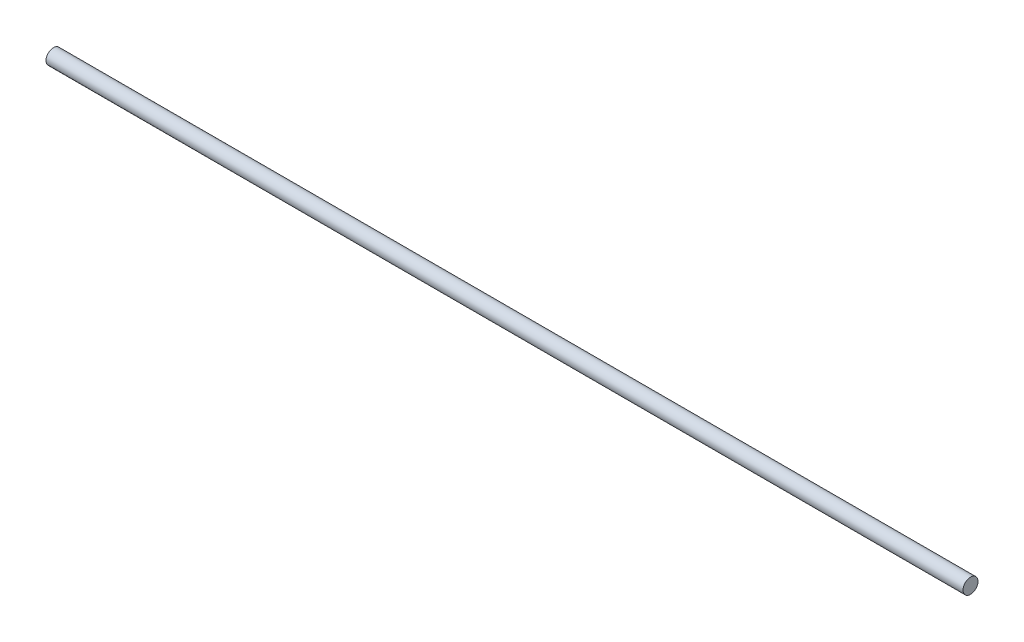
SolidWorks part; units mm, degrees
material "Plain carbon steel"
ref_plane "Front Plane" through (0, 0, 0) normal (0, 0, 1) x (1, 0, 0)
ref_plane "Top Plane" through (0, 0, 0) normal (0, 1, 0) x (1, 0, 0)
ref_plane "Right Plane" through (0, 0, 0) normal (1, 0, 0) x (0, 0, -1)
sketch "Sketch1" plane through (0, 0, 0) normal (0, 0, 1) x (1, 0, 0)
  line L0 (-202.6045, 0) -> (262.3615, 0) construction
  line L1 (-767, 0) -> (-767, 12.5)
  line L2 (-767, 12.5) -> (0, 12.5)
  line L3 (0, 12.5) -> (0, 0)
  line L6 (0, 0) -> (-767, 0)
  dimension "D1" = 767
  dimension "D4" = 12.5
revolve "Revolve1" add sketch "Sketch1" angle 360 about L0
sketch "Sketch3" plane through (-767, 0, 0) normal (-1, 0, 0) x (0, 0, 1)
  line L2 (-6, 10.9659) -> (-6, -10.9659)
  line L4 (6, 10.9659) -> (6, -10.9659)
  arc A0 (-6, 10.9659) -> (-6, -10.9659) centre (0, 0) ccw
  circle A1 centre (0, 0) radius 12.5
  arc A2 (6, -10.9659) -> (6, 10.9659) centre (0, 0) ccw
  dimension "D2" = 12
  dimension "D3" = 6
  dimension "D1" = 0
extrude "Cut-Extrude1" [suppressed] cut sketch "Sketch3" against normal blind 17
mirror "Mirror1" about plane through (0, 0, 0) normal (1, 0, 0) of "Cut-Extrude1", "Revolve1"
